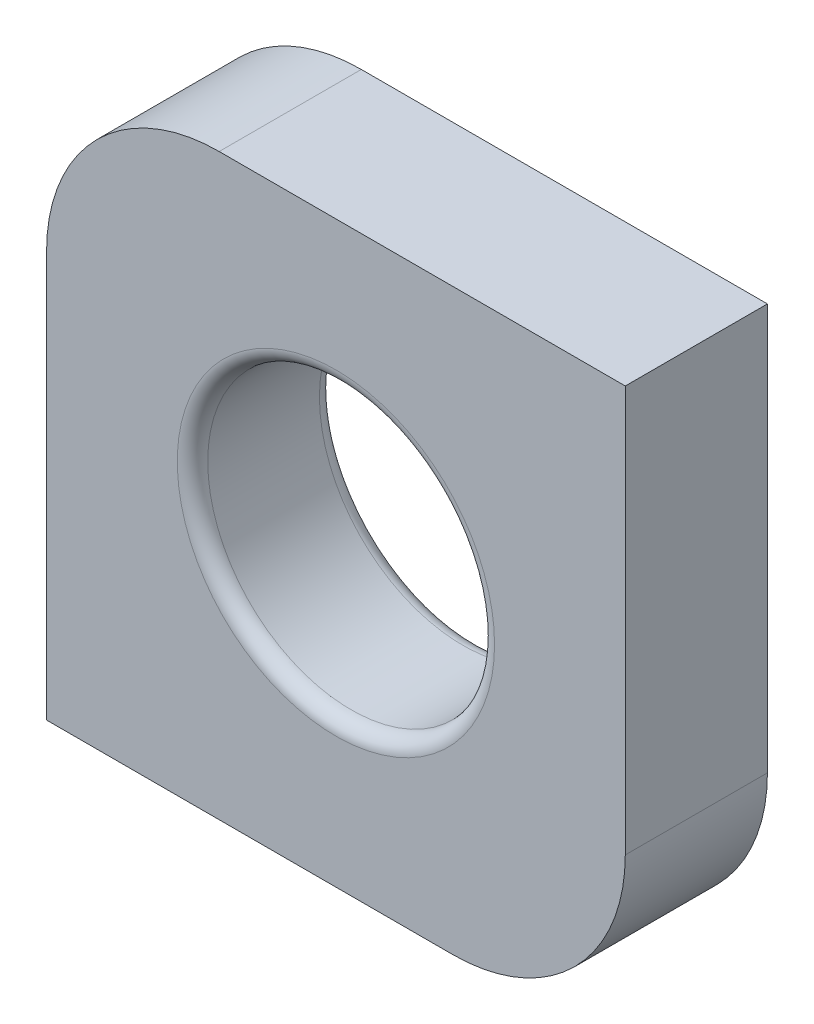
from build123d import *

# Parameters (mm, degrees)
SKETCH1_W           = 114
SKETCH1_H           = 114
SKETCH1_R           = 28.25
BOSS_EXTRUDE1_DEPTH = 28
FILLET1_R           = 3
FILLET3_R           = 34


with BuildPart() as part:
    # Sketch1 → Boss-Extrude1 (new body)
    with BuildSketch(Plane.XY):
        Rectangle(SKETCH1_W, SKETCH1_H)
        Circle(SKETCH1_R, mode=Mode.SUBTRACT)
    extrude(amount=BOSS_EXTRUDE1_DEPTH)

    # Fillet1
    fillet1_edges = [part.edges().sort_by_distance(p)[0] for p in [
        (-28.25, 0, 0),
        (-28.25, 0, 28),
    ]]
    fillet(fillet1_edges, radius=FILLET1_R)

    # Fillet3
    fillet3_edges = [part.edges().sort_by_distance(p)[0] for p in [
        (-57, 57, 14),
        (57, -57, 14),
    ]]
    fillet(fillet3_edges, radius=FILLET3_R)


solid = part.part
